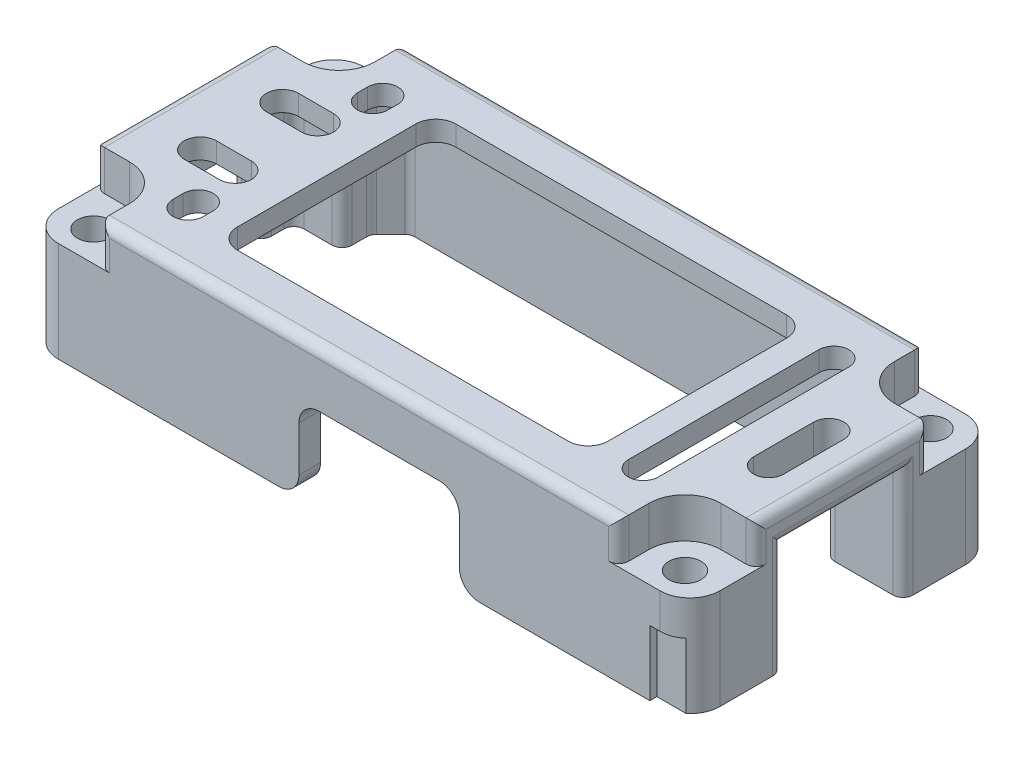
from build123d import *

# Parameters (mm, degrees)
SKETCH_1_R           = 1.6
EXTRUDE_1_DEPTH      = 12
SKETCH_2_W           = 52
SKETCH_2_H           = 26.2
CUT_EXTRUDE_1_DEPTH  = 2
SKETCH_3_W           = 7.4
SKETCH_3_H           = 20
CUT_EXTRUDE_2_DEPTH  = 8
SKETCH_4_W           = 16
SKETCH_4_H           = 4.5
CUT_EXTRUDE_3_DEPTH  = 2.15
SKETCH_5_W           = 52
SKETCH_5_H           = 26.2
CUT_EXTRUDE_4_DEPTH  = 39.28266579
SKETCH_6_W           = 66
SKETCH_6_H           = 30.5
SKETCH_6_R           = 1.6
SKETCH_6_W_2         = 37
SKETCH_6_H_2         = 21.8
EXTRUDE_2_DEPTH      = 2
SKETCH_7_W           = 2
SKETCH_7_H           = 12
SKETCH_7_W_2         = 1.6
SKETCH_7_H_2         = 8
CUT_EXTRUDE_5_DEPTH  = 39.28266579
SKETCH_8_W           = 16
SKETCH_8_H           = 2.15
CUT_EXTRUDE_6_DEPTH  = 38.33379836
SKETCH_9_W           = 0.8
SKETCH_9_H           = 7.1
EXTRUDE_3_DEPTH      = 12
CUT_EXTRUDE_7_DEPTH  = 12
SKETCH_11_W          = 3
SKETCH_11_H          = 10
EXTRUDE_4_DEPTH      = 3
SKETCH_13_W          = 7.8
SKETCH_13_H          = 12
EXTRUDE_5_DEPTH      = 1
CHAMFER_1_SIZE       = 2
CUT_EXTRUDE_8_DEPTH  = 4
CUT_EXTRUDE_9_DEPTH  = 39.955904559
FILLET_R1_R          = 1
FILLET_R2_R          = 2
FILLET_R3_R          = 3
CUT_EXTRUDE_START    = -6.5
CUT_EXTRUDE_10_DEPTH = 6.5


with BuildPart() as part:
    # 草图1 → 凸台-拉伸1 (new body)
    with BuildSketch(Plane(origin=(0, 0, 0), x_dir=(1, 0, 0), z_dir=(0, 1, 0))):
        Polygon((-33, 4), (-27.6, 4), (-27.6, -4), (-33, -4), (-33, -15.25), (33, -15.25), (33, -6), (28, -6), (28, 6), (33, 6), (33, 15.25), (-33, 15.25), align=None)
        with Locations(Location((-29.5, 12.25, 0), (0, 0, 270))):
            Circle(SKETCH_1_R, mode=Mode.SUBTRACT)
        with Locations(Location((29.5, 12.25, 0), (0, 0, 270))):
            Circle(SKETCH_1_R, mode=Mode.SUBTRACT)
        with Locations(Location((-29.5, -12.25, 0), (0, 0, 90))):
            Circle(SKETCH_1_R, mode=Mode.SUBTRACT)
        with Locations(Location((29.5, -12.25, 0), (0, 0, 90))):
            Circle(SKETCH_1_R, mode=Mode.SUBTRACT)
        Polygon((-26, -5.75), (-26, 5.75), (-21.1, 5.75), (-21.1, 13.1), (21.1, 13.1), (21.1, -13.1), (-21.1, -13.1), (-21.1, -5.75), align=None, mode=Mode.SUBTRACT)
    extrude(amount=EXTRUDE_1_DEPTH)

    # 草图2 → 切除-拉伸1 (cut)
    with BuildSketch(Plane.XZ):
        Rectangle(SKETCH_2_W, SKETCH_2_H)
    extrude(amount=-CUT_EXTRUDE_1_DEPTH, mode=Mode.SUBTRACT)

    # 草图3 → 切除-拉伸2 (cut)
    with BuildSketch(Plane(origin=(0, 12, 0), x_dir=(1, 0, 0), z_dir=(0, 1, 0))):
        with Locations((-26.8, 0)):
            Rectangle(SKETCH_3_W, SKETCH_3_H)
        Polygon((28, -6), (28, 6), (26, 6), (26, 13.1), (21.1, 13.1), (21.1, -13.1), (26, -13.1), (26, -6), align=None)
    extrude(amount=-CUT_EXTRUDE_2_DEPTH, mode=Mode.SUBTRACT)

    # 草图4 → 切除-拉伸3 (cut)
    with BuildSketch(Plane.XY.offset(15.25)):
        with Locations((2, 6.25)):
            Rectangle(SKETCH_4_W, SKETCH_4_H)
    extrude(amount=-CUT_EXTRUDE_3_DEPTH, mode=Mode.SUBTRACT)

    # 草图5 → 切除-拉伸4 (cut, through all)
    with BuildSketch(Plane.XZ):
        Rectangle(SKETCH_5_W, SKETCH_5_H)
    extrude(amount=-CUT_EXTRUDE_4_DEPTH, mode=Mode.SUBTRACT)

    # 草图6 → 凸台-拉伸2 (add)
    with BuildSketch(Plane(origin=(0, 12, 0), x_dir=(1, 0, 0), z_dir=(0, 1, 0))):
        Rectangle(SKETCH_6_W, SKETCH_6_H)
        with Locations(Location((-29.5, -12.25, 0), (0, 0, 90))):
            Circle(SKETCH_6_R, mode=Mode.SUBTRACT)
        with Locations(Location((29.5, -12.25, 0), (0, 0, 90))):
            Circle(SKETCH_6_R, mode=Mode.SUBTRACT)
        with Locations(Location((29.5, 12.25, 0), (0, 0, 270))):
            Circle(SKETCH_6_R, mode=Mode.SUBTRACT)
        with Locations(Location((-29.5, 12.25, 0), (0, 0, 270))):
            Circle(SKETCH_6_R, mode=Mode.SUBTRACT)
        Rectangle(SKETCH_6_W_2, SKETCH_6_H_2, mode=Mode.SUBTRACT)
    extrude(amount=EXTRUDE_2_DEPTH)

    # 草图7 → 切除-拉伸5 (cut, through all)
    with BuildSketch(Plane.XZ.offset(-12)):
        with Locations((27, 0)):
            Rectangle(SKETCH_7_W, SKETCH_7_H)
        with Locations((-26.8, 0)):
            Rectangle(SKETCH_7_W_2, SKETCH_7_H_2)
    extrude(amount=CUT_EXTRUDE_5_DEPTH, mode=Mode.SUBTRACT)

    # 草图8 → 切除-拉伸6 (cut, through all)
    with BuildSketch(Plane.XZ.offset(-8.5)):
        with Locations((2, 14.175)):
            Rectangle(SKETCH_8_W, SKETCH_8_H)
    extrude(amount=CUT_EXTRUDE_6_DEPTH, mode=Mode.SUBTRACT)

    # 草图9 → 凸台-拉伸3 (add, through all)
    with BuildSketch(Plane.XZ.offset(-12)):
        with Locations((25.6, 9.55)):
            Rectangle(SKETCH_9_W, SKETCH_9_H)
        Polygon((-25.2, -13.1), (-26, -13.1), (-26, -10), (-30.5, -10), (-30.5, -4), (-33, -4), (-33, 4), (-30.5, 4), (-30.5, 10), (-26, 10), (-26, 13.1), (-25.2, 13.1), align=None)
        with Locations((25.6, -9.55)):
            Rectangle(SKETCH_9_W, SKETCH_9_H)
    extrude(amount=EXTRUDE_3_DEPTH)

    # 草图10 → 切除-拉伸7 (cut)
    with BuildSketch(Plane.XZ):
        Polygon((-33, -5), (-33, 5), (-30, 5), (-30, 8.25), (-25.2, 8.25), (-25.2, -8.25), (-30, -8.25), (-30, -5), align=None)
    extrude(amount=-CUT_EXTRUDE_7_DEPTH, mode=Mode.SUBTRACT)

    # 草图11 → 凸台-拉伸4 (add)
    with BuildSketch(Plane.XZ.offset(-12)):
        with Locations((-31.5, 0)):
            Rectangle(SKETCH_11_W, SKETCH_11_H)
    extrude(amount=EXTRUDE_4_DEPTH)

    # 草图13 → 凸台-拉伸5 (add)
    with BuildSketch(Plane.XZ.offset(-12)):
        with Locations((29.1, 0)):
            Rectangle(SKETCH_13_W, SKETCH_13_H)
    extrude(amount=EXTRUDE_5_DEPTH)

    # 倒角1
    chamfer_1_edges = [part.edges().sort_by_distance(p)[0] for p in [
        (-25.2, 6, -13.1),
        (-25.2, 6, 13.1),
        (25.2, 6, 13.1),
        (25.2, 6, -13.1),
    ]]
    chamfer(chamfer_1_edges, length=CHAMFER_1_SIZE)

    # 草图12 → 切除-拉伸8 (cut)
    with BuildSketch(Plane(origin=(0, 14, 0), x_dir=(1, 0, 0), z_dir=(0, 1, 0))):
        with BuildLine():
            Line((-29.5, 8.65), (-33, 8.65))
            Line((-33, 8.65), (-33, 15.25))
            Line((-33, 15.25), (-25.9, 15.25))
            Line((-25.9, 15.25), (-25.9, 12.25))
            ThreePointArc((-25.9, 12.25), (-26.954415588, 9.704415588), (-29.5, 8.65))
        make_face()
        with BuildLine():
            Line((29.5, 8.65), (33, 8.65))
            Line((33, 8.65), (33, 15.25))
            Line((33, 15.25), (25.9, 15.25))
            Line((25.9, 15.25), (25.9, 12.25))
            ThreePointArc((25.9, 12.25), (26.954415588, 9.704415588), (29.5, 8.65))
        make_face()
        with BuildLine():
            Line((29.5, -8.65), (33, -8.65))
            Line((33, -8.65), (33, -15.25))
            Line((33, -15.25), (25.9, -15.25))
            Line((25.9, -15.25), (25.9, -12.25))
            ThreePointArc((25.9, -12.25), (26.954415588, -9.704415588), (29.5, -8.65))
        make_face()
        with BuildLine():
            Line((-25.9, -12.25), (-25.9, -15.25))
            Line((-25.9, -15.25), (-33, -15.25))
            Line((-33, -15.25), (-33, -8.65))
            Line((-33, -8.65), (-29.5, -8.65))
            ThreePointArc((-29.5, -8.65), (-26.954415588, -9.704415588), (-25.9, -12.25))
        make_face()
    extrude(amount=-CUT_EXTRUDE_8_DEPTH, mode=Mode.SUBTRACT)

    # 草图14 → 切除-拉伸9 (cut, through all)
    with BuildSketch(Plane(origin=(0, 14, 0), x_dir=(1, 0, 0), z_dir=(0, 1, 0))):
        with BuildLine():
            Line((21.1, -9.5), (21.1, 9.5))
            ThreePointArc((21.1, 9.5), (22.6, 11), (24.1, 9.5))
            Line((24.1, 9.5), (24.1, -9.5))
            ThreePointArc((24.1, -9.5), (22.6, -11), (21.1, -9.5))
        make_face()
        with BuildLine():
            Line((27.1, -3), (27.1, 3))
            ThreePointArc((27.1, 3), (28.6, 4.5), (30.1, 3))
            Line((30.1, 3), (30.1, -3))
            ThreePointArc((30.1, -3), (28.6, -4.5), (27.1, -3))
        make_face()
        with BuildLine():
            Line((-27, 5.7), (-23.5, 5.7))
            ThreePointArc((-23.5, 5.7), (-21.9, 4.1), (-23.5, 2.5))
            Line((-23.5, 2.5), (-27, 2.5))
            ThreePointArc((-27, 2.5), (-28.6, 4.1), (-27, 5.7))
        make_face()
        with BuildLine():
            Line((-27, -5.7), (-23.5, -5.7))
            ThreePointArc((-23.5, -5.7), (-21.9, -4.1), (-23.5, -2.5))
            Line((-23.5, -2.5), (-27, -2.5))
            ThreePointArc((-27, -2.5), (-28.6, -4.1), (-27, -5.7))
        make_face()
        with BuildLine():
            Line((-21.1, 9.7), (-21.1, 8.7))
            ThreePointArc((-21.1, 8.7), (-22.6, 7.2), (-24.1, 8.7))
            Line((-24.1, 8.7), (-24.1, 9.7))
            ThreePointArc((-24.1, 9.7), (-22.6, 11.2), (-21.1, 9.7))
        make_face()
        with BuildLine():
            Line((-21.1, -9.7), (-21.1, -8.7))
            ThreePointArc((-21.1, -8.7), (-22.6, -7.2), (-24.1, -8.7))
            Line((-24.1, -8.7), (-24.1, -9.7))
            ThreePointArc((-24.1, -9.7), (-22.6, -11.2), (-21.1, -9.7))
        make_face()
    extrude(amount=-CUT_EXTRUDE_9_DEPTH, mode=Mode.SUBTRACT)

    # R1 过渡圆角
    fillet_r1_edges = [part.edges().sort_by_distance(p)[0] for p in [
        (25.2, 5.5, 6),
        (25.2, 5.5, -6),
        (-30, 6, -8.25),
        (-25.2, 6, -8.25),
        (-25.2, 6, 8.25),
        (-30, 6, 8.25),
        (-30, 4.5, 5),
        (-33, 4.5, 5),
        (-30, 4.5, -5),
        (-33, 4.5, -5),
        (-33, 9, 0),
        (33, 5.5, 6),
        (33, 5.5, -6),
        (33, 11, 0),
        (-25.2, 6, -11.1),
        (23.2, 6, -13.1),
        (-23.2, 6, -13.1),
        (25.2, 6, 11.1),
        (25.2, 6, -11.1),
        (-23.2, 6, 13.1),
        (23.2, 6, 13.1),
        (-25.2, 6, 11.1),
        (0, 14, -15.25),
        (-33, 14, 0),
        (0, 14, 15.25),
        (33, 14, 0),
        (33, 12, 8.65),
        (25.9, 12, 15.25),
        (-25.9, 12, 15.25),
        (-33, 12, 8.65),
        (-33, 12, -8.65),
        (-25.9, 12, -15.25),
        (25.9, 12, -15.25),
        (33, 12, -8.65),
    ]]
    fillet(fillet_r1_edges, radius=FILLET_R1_R)

    # R2 过渡圆角
    fillet_r2_edges = [part.edges().sort_by_distance(p)[0] for p in [
        (10, 8.5, 14.175),
        (-6, 8.5, 14.175),
        (-18.5, 13, 10.9),
        (18.5, 13, 10.9),
        (18.5, 13, -10.9),
        (-18.5, 13, -10.9),
        (10, 0, 14.175),
        (-6, 0, 14.175),
    ]]
    fillet(fillet_r2_edges, radius=FILLET_R2_R)

    # R3 过渡圆角
    fillet_r3_edges = [part.edges().sort_by_distance(p)[0] for p in [
        (-33, 5, 15.25),
        (-33, 5, -15.25),
        (33, 5, -15.25),
        (33, 5, 15.25),
    ]]
    fillet(fillet_r3_edges, radius=FILLET_R3_R)

    # 草图15 → 切除-拉伸10 (cut)
    with BuildSketch(Plane.XZ.offset(CUT_EXTRUDE_START)):
        with BuildLine():
            Line((29, 15.25), (30, 15.25))
            ThreePointArc((30, 15.25), (31.024695077, 15.069574436), (31.926136028, 14.55))
            Line((31.926136028, 14.55), (29, 14.55))
            Line((29, 14.55), (29, 15.25))
        make_face()
    extrude(amount=CUT_EXTRUDE_10_DEPTH, mode=Mode.SUBTRACT)


solid = part.part
